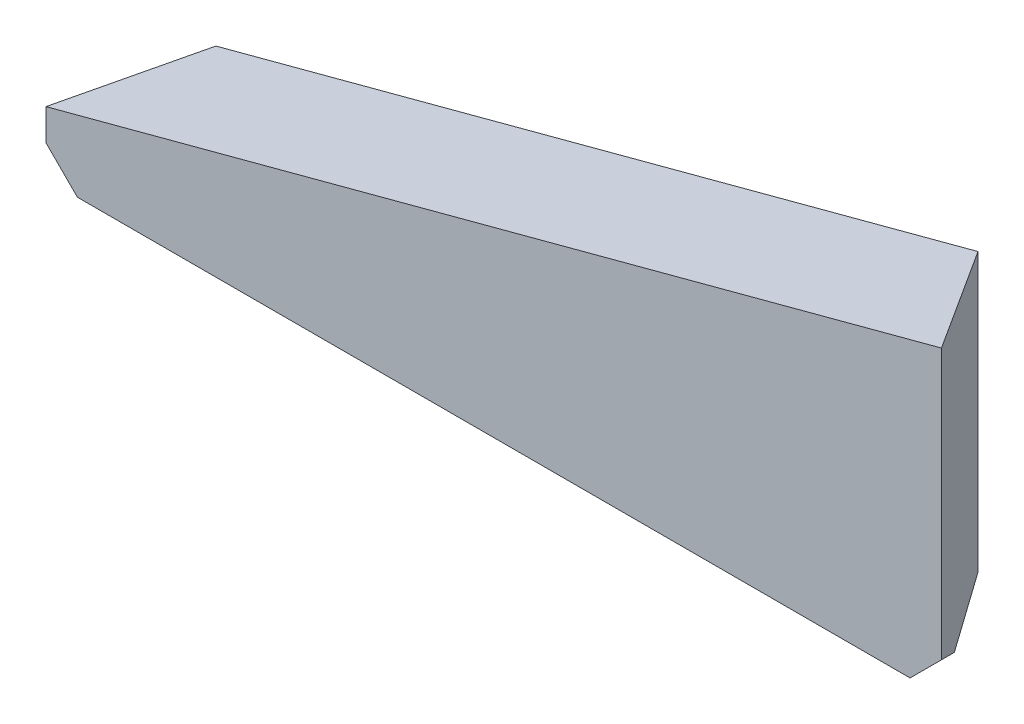
SolidWorks part; units mm, degrees
ref_plane "Front Plane" through (0, 0, 0) normal (0, 0, 1) x (1, 0, 0)
ref_plane "Top Plane" through (0, 0, 0) normal (0, 1, 0) x (1, 0, 0)
ref_plane "Right Plane" through (0, 0, 0) normal (1, 0, 0) x (0, 0, -1)
sketch "Sketch1" plane through (0, 0, 0) normal (0, 0, 1) x (1, 0, 0)
  line L0 (5, 0) -> (137.6, 0)
  line L1 (142.6, 5) -> (142.6, 48)
  line L2 (142.6, 48) -> (0, 10)
  line L3 (0, 10) -> (0, 5)
  line L4 (0, 5) -> (5, 0)
  line L5 (137.6, 0) -> (142.6, 5)
  point P0 (0, 0)
  point P1 (142.6, 0)
  dimension "D1" = 10
  dimension "D2" = 48
  dimension "D3" = 142.6
extrude "Boss-Extrude1" add sketch "Sketch1" along normal blind 20
sketch "Sketch2" plane through (-2.4881, 9.337, 0) normal (-0.2575, 0.9663, 0) x (0.9663, 0.2575, 0)
  line L0 (2.5749, -20) -> (9.8749, 0)
  line L1 (150.1512, 0) -> (2.5749, 0) construction
  line L2 (150.1512, -20) -> (135.4749, 0)
  line L3 (150.1512, -20) -> (150.1512, 0) construction
  line L4 (150.1512, -20) -> (150.1512, 0)
  line L5 (2.5749, -20) -> (2.5749, 0) construction
  line L6 (2.5749, -20) -> (2.5749, 0)
  line L7 (150.1512, 0) -> (135.4749, 0)
  line L8 (9.8749, 0) -> (2.5749, 0)
  dimension "D1" = 7.3
  dimension "D2" = 125.6
extrude "Cut-Extrude2" cut sketch "Sketch2" along direction (0, 1, 0) on the side against the normal blind 50
